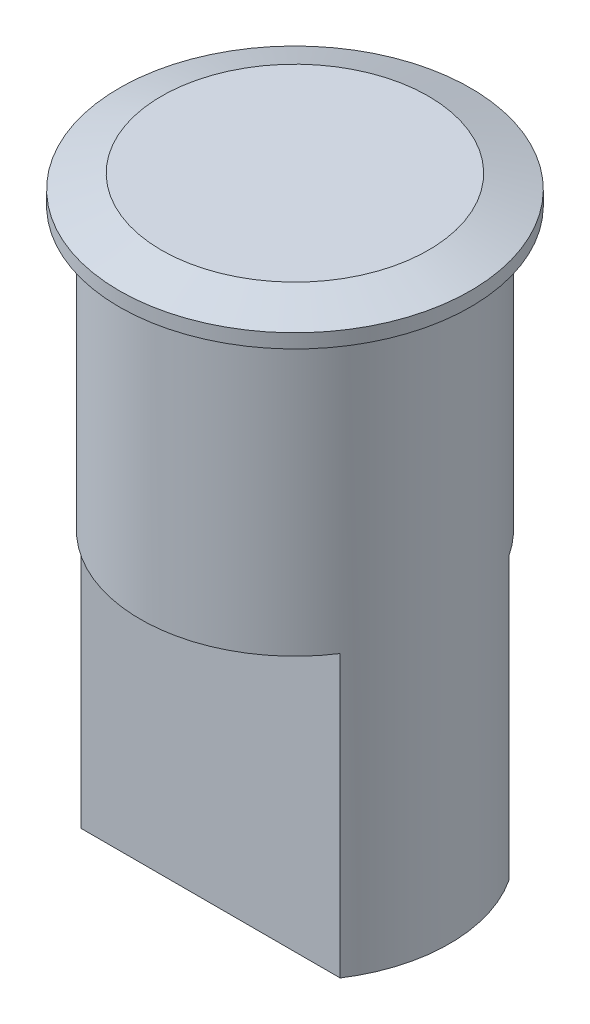
SolidWorks part; units mm, degrees
material "6061"
ref_plane "前视基准面" through (0, 0, 0) normal (0, 0, 1) x (1, 0, 0)
ref_plane "上视基准面" through (0, 0, 0) normal (0, 1, 0) x (1, 0, 0)
ref_plane "右视基准面" through (0, 0, 0) normal (1, 0, 0) x (0, 0, -1)
sketch "草图1" plane through (0, 0, 0) normal (0, 1, 0) x (1, 0, 0)
  circle A0 centre (0, 0) radius 11
  dimension "D1" = 22
extrude "凸台-拉伸1" add sketch "草图1" along normal blind 20
sketch "草图2" plane through (0, 0, 0) normal (0, -1, 0) x (1, 0, 0)
  line L1 (-9.2195, 6) -> (9.2195, 6)
  line L2 (-9.2195, 6) -> (-9.2195, -6)
  line L3 (-9.2195, -6) -> (9.2195, -6)
  line L4 (9.2195, 6) -> (9.2195, -6)
  line L5 (-9.2195, 6) -> (9.2195, -6) construction
  line L6 (-9.2195, -6) -> (9.2195, 6) construction
  circle A0 centre (0, 0) radius 11 construction
  circle A1 centre (0, 0) radius 11
  point P0 (0, 0)
  circle M3 centre (0, 0) radius 11
  dimension "D1" = 12
extrude "凸台-拉伸2" add sketch "草图2" along normal blind 20 contours L2 M3 | L4 L1 L2 L3 | L4 M3
sketch "草图3" plane through (0, 20, 0) normal (0, 1, 0) x (1, 0, 0)
  circle A0 centre (0, 0) radius 12.5
  dimension "D1" = 25
extrude "凸台-拉伸3" add sketch "草图3" along normal blind 2
chamfer "倒角1" distance 1 distance2 3 1 edges at (0, 22, 12.5)
